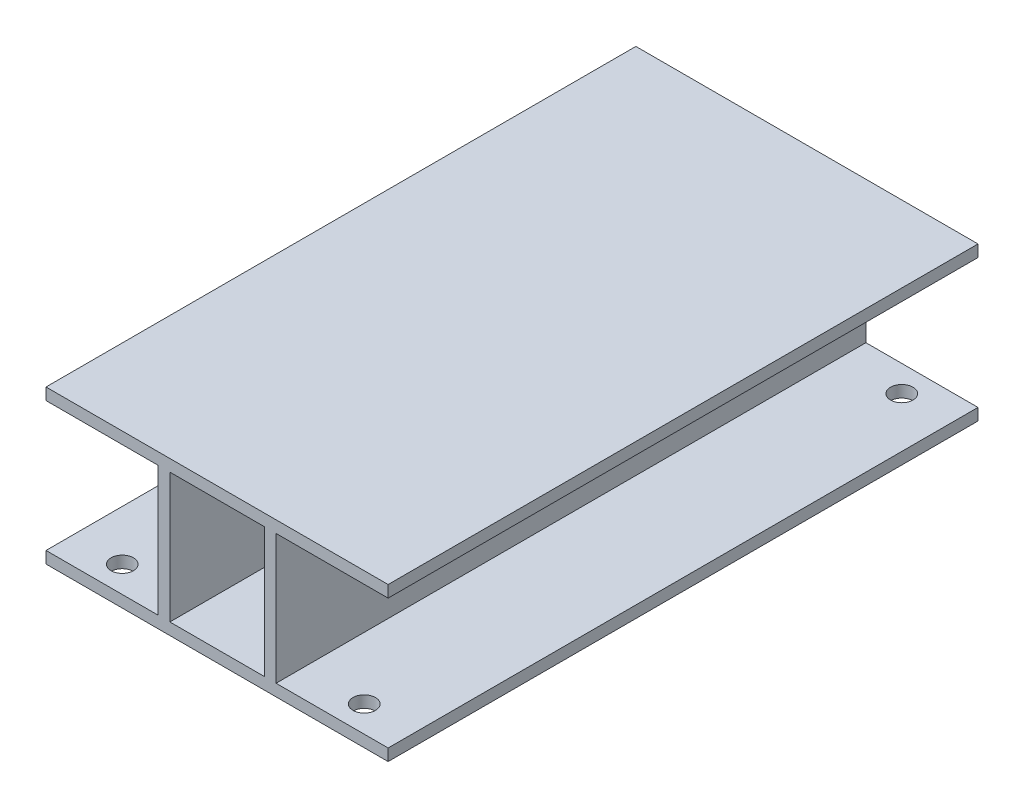
SolidWorks part; units mm, degrees
ref_plane "Front Plane" through (0, 0, 0) normal (0, 0, 1) x (1, 0, 0)
ref_plane "Top Plane" through (0, 0, 0) normal (0, 1, 0) x (1, 0, 0)
ref_plane "Right Plane" through (0, 0, 0) normal (1, 0, 0) x (0, 0, -1)
other "Configuration Table"
sketch "Sketch1" plane through (0, 0, 0) normal (0, 0, 1) x (1, 0, 0)
  line L0 (0, 0) -> (0, 260) construction
  line L13 (-290, 260) -> (290, 260)
  line L14 (290, 260) -> (290, 240)
  line L15 (290, 240) -> (100, 240)
  line L16 (100, 240) -> (100, 20)
  line L17 (100, 20) -> (290, 20)
  line L18 (290, 20) -> (290, 0)
  line L19 (290, 0) -> (-290, 0)
  line L20 (-80, 240) -> (80, 240)
  line L21 (80, 240) -> (80, 20)
  line L22 (80, 20) -> (-80, 20)
  line L23 (-80, 240) -> (-80, 20)
  line L24 (-290, 20) -> (-290, 0)
  line L25 (-100, 20) -> (-290, 20)
  line L26 (-100, 240) -> (-100, 20)
  line L27 (-290, 240) -> (-100, 240)
  line L28 (-290, 260) -> (-290, 240)
  point P14 (0, 20)
  point P15 (0, 240)
  dimension "D1" = 260
  dimension "D2" = 20
  dimension "D3" = 20
  dimension "D4" = 160
  dimension "D5" = 20
  dimension "D6" = 580
extrude "Boss-Extrude1" add sketch "Sketch1" along normal blind 1000
sketch "Sketch2" plane through (0, 0, 0) normal (0, -1, 0) x (-1, 0, 0)
  line L0 (-290, -500) -> (290, -500) construction
  line L1 (205.1242, -955.6395) -> (-205.1242, -955.6395) construction
  line L2 (205.1242, -955.6395) -> (205.1242, -44.3605) construction
  line L3 (205.1242, -44.3605) -> (-205.1242, -44.3605) construction
  line L4 (-205.1242, -955.6395) -> (-205.1242, -44.3605) construction
  line L5 (205.1242, -955.6395) -> (-205.1242, -44.3605) construction
  line L6 (205.1242, -44.3605) -> (-205.1242, -955.6395) construction
  line L7 (-290, -1000) -> (-290, 0) construction
  line L8 (290, -1000) -> (290, 0) construction
  line L9 (0, -1000) -> (0, 0) construction
  line L10 (290, -1000) -> (-290, -1000) construction
  circle A0 centre (205.1242, -955.6395) radius 19
  circle A1 centre (-205.1242, -955.6395) radius 19
  circle A2 centre (-205.1242, -44.3605) radius 19
  circle A3 centre (205.1242, -44.3605) radius 19
  point P0 (0, -500)
  dimension "D1" = 38
extrude "Cut-Extrude1" cut sketch "Sketch2" against normal blind 30
